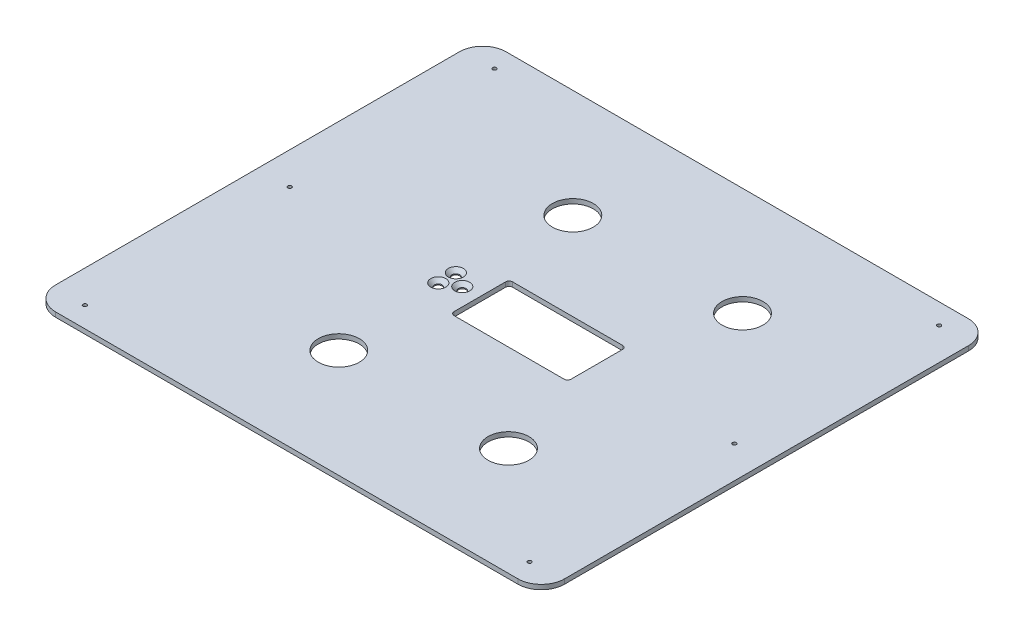
SolidWorks part; units mm, degrees
material "Plain Carbon Steel"
ref_plane "Front Plane" through (0, 0, 0) normal (0, 0, 1) x (1, 0, 0)
ref_plane "Top Plane" through (0, 0, 0) normal (0, 1, 0) x (1, 0, 0)
ref_plane "Right Plane" through (0, 0, 0) normal (1, 0, 0) x (0, 0, -1)
sketch "Sketch1" plane through (0, 0, 0) normal (0, 1, 0) x (1, 0, 0)
  line L1 (-217.5, -192.5) -> (217.5, -192.5)
  line L2 (-217.5, -192.5) -> (-217.5, 192.5)
  line L3 (-217.5, 192.5) -> (217.5, 192.5)
  line L4 (217.5, -192.5) -> (217.5, 192.5)
  line L5 (-217.5, -192.5) -> (217.5, 192.5) construction
  line L6 (-217.5, 192.5) -> (217.5, -192.5) construction
  point P0 (0, 0)
  dimension "D1" = 385
  dimension "D2" = 435
extrude "Boss-Extrude1" add sketch "Sketch1" along normal blind 4
fillet "Fillet1" radius 20 4 edges at (-217.5, 2, 192.5) (-217.5, 2, -192.5) (217.5, 2, -192.5) (217.5, 2, 192.5)
sketch "Sketch2" plane through (0, 4, 0) normal (0, 1, 0) x (1, 0, 0)
  circle A0 centre (-42.5, 0) radius 1.5555
  circle A1 centre (-55.5, 7.5) radius 1.5
  circle A2 centre (-55.5, -7.5) radius 1.9249
  dimension "D1" = 3.1109
  dimension "D2" = 3
  dimension "D3" = 3.8497
extrude "Cut-Extrude1" cut sketch "Sketch2" against normal blind 10
sketch "Sketch3" plane through (0, 4, 0) normal (0, 1, 0) x (1, 0, 0)
  line L0 (-27.5, 20) -> (-27.5, -20) construction
  line L1 (-24.5, -25) -> (69.5, -25)
  line L2 (-27.5, -22) -> (-27.5, 22)
  line L3 (-24.5, 25) -> (69.5, 25)
  line L4 (72.5, -22) -> (72.5, 22)
  line L5 (-27.5, -25) -> (72.5, 25) construction
  line L6 (-27.5, 25) -> (72.5, -25) construction
  arc A0 (-24.5, -25) -> (-27.5, -22) centre (-24.5, -22) cw
  arc A1 (69.5, -25) -> (72.5, -22) centre (69.5, -22) ccw
  arc A2 (69.5, 25) -> (72.5, 22) centre (69.5, 22) cw
  arc A3 (-27.5, 22) -> (-24.5, 25) centre (-24.5, 22) cw
  point P0 (22.5, 0)
  dimension "D3" = 3
  dimension "D1" = 100
  dimension "D2" = 50
extrude "Cut-Extrude2" cut sketch "Sketch3" against normal blind 4
hole_wizard "Hole Size (% by) Hexalobular Countersunk Head Screw Type1" positions "Sketch4" profile "Sketch5" countersink size "M6" standard "GB"
sketch "Sketch4" plane through (0, 4, 0) normal (0, 1, 0) x (1, 0, 0)
  point P0 (-55.5, -7.5)
  point P3 (-42.5, 0)
  point P6 (-55.5, 7.5)
sketch "Sketch5" plane through (-55.5, 4, 7.5) normal (1, 0, 0) x (0, 0, 1)
  line L0 (0, 0) -> (0, 9.4828)
  line L1 (0, 9.4828) -> (3.3, 7.5)
  line L2 (3.3, 7.5) -> (3.3, 3.1)
  line L3 (3.3, 3.1) -> (6.4, 0)
  line L5 (6.4, 0) -> (0, 0)
  line L6 (-3.3, 3.1) -> (-6.4, 0) construction
  line L10 (0, 9.4828) -> (-3.3, 7.5) construction
  line L11 (0, -6.35) -> (0, 107.95) construction
  dimension "孔直径" = 6.6
  dimension "孔深度" = 7.5
  dimension "近端锥形沉头孔直径" = 12.8
  dimension "近端锥形沉头孔角度" = 90
  dimension "导头角度" = 118
sketch "Sketch6" plane through (0, 0, 0) normal (0, -1, 0) x (1, 0, 0)
  circle A0 centre (-48, 100) radius 17.5
  circle A1 centre (97, 100) radius 17.5
  circle A2 centre (-48, -100) radius 17.5
  circle A3 centre (97, -100) radius 17.5
  dimension "D1" = 35
extrude "Cut-Extrude3" cut sketch "Sketch6" against normal blind 4
sketch "Sketch7" plane through (0, 0, 0) normal (0, -1, 0) x (1, 0, 0)
  line L1 (-190, -175) -> (190, -175) construction
  line L2 (-190, -175) -> (-190, 175) construction
  line L3 (-190, 175) -> (190, 175) construction
  line L4 (190, -175) -> (190, 175) construction
  line L5 (-190, -175) -> (190, 175) construction
  line L6 (-190, 175) -> (190, -175) construction
  circle A0 centre (-190, 175) radius 1.6
  circle A1 centre (-190, 0) radius 1.6
  circle A2 centre (-190, -175) radius 1.6
  circle A3 centre (190, 175) radius 1.6
  circle A4 centre (190, 0) radius 1.6
  circle A5 centre (190, -175) radius 1.6
  point P0 (0, 0)
  dimension "D3" = 3.2
  dimension "D1" = 380
  dimension "D2" = 350
extrude "Cut-Extrude4" cut sketch "Sketch7" against normal blind 4
